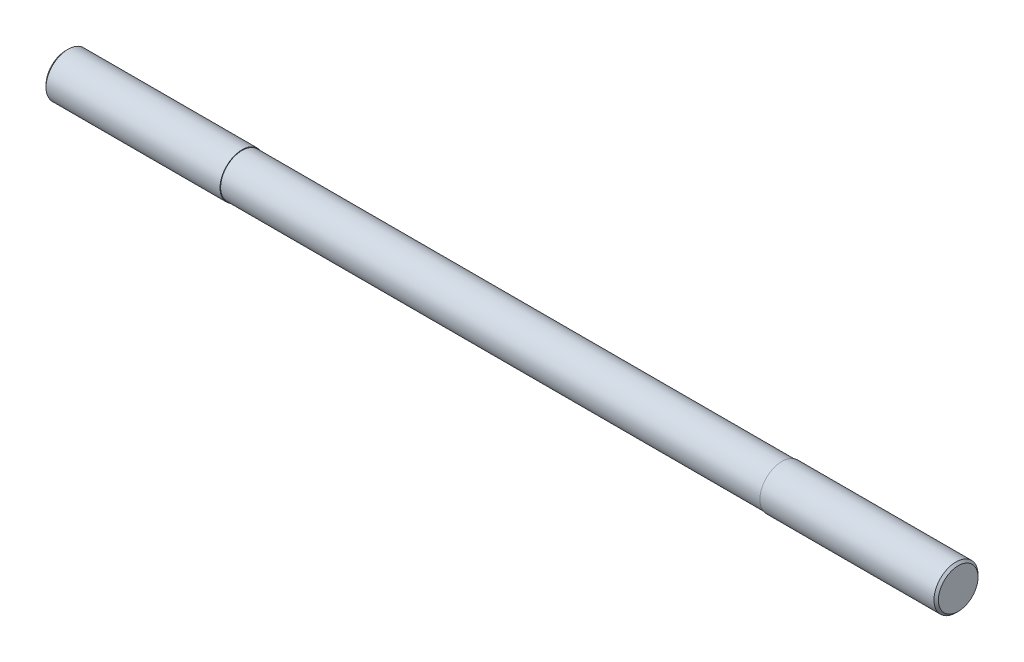
from build123d import *

# Parameters (mm, degrees)
CHAMFER1_SIZE = 1


with BuildPart() as part:
    # Sketch3 → Revolve1 (revolve)
    with BuildSketch(Plane.XY, mode=Mode.PRIVATE) as revolve1_sk:
        Polygon((325, 10), (405, 10), (405, 0), (0, 0), (0, 10), (80, 10), (80, 9.75), (325, 9.75), align=None)
    revolve(revolve1_sk.sketch.rotate(Axis((0, 0, 0), (1, 0, 0)), 90), axis=Axis((0, 0, 0), (1, 0, 0)))

    # Chamfer1
    chamfer1_edges = [part.edges().sort_by_distance(p)[0] for p in [
        (405, 0, -10),
        (0, 0, -10),
    ]]
    chamfer(chamfer1_edges, length=CHAMFER1_SIZE)


solid = part.part
